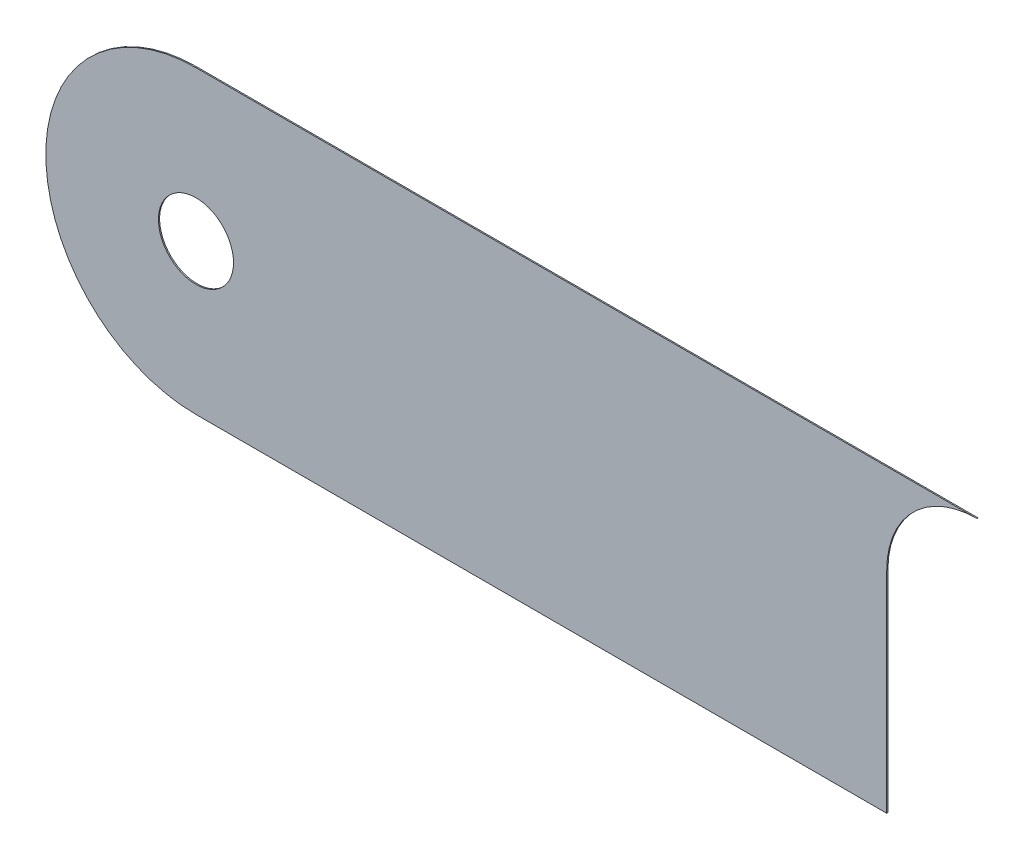
SolidWorks part; units mm, degrees
material "普通碳钢"
ref_plane "Front Plane" through (0, 0, 0) normal (0, 0, 1) x (1, 0, 0)
ref_plane "Top Plane" through (0, 0, 0) normal (0, 1, 0) x (1, 0, 0)
ref_plane "Right Plane" through (0, 0, 0) normal (1, 0, 0) x (0, 0, -1)
sketch "Sketch1" plane through (0, 0, 0) normal (0, 0, 1) x (1, 0, 0)
  line L0 (0, 254) -> (1320.8, 254)
  line L1 (0, -254) -> (1168.4, -254)
  line L2 (1168.4, -254) -> (1168.4, 101.6)
  circle A0 centre (0, 0) radius 63.5
  arc A1 (0, 254) -> (0, -254) centre (0, 0) ccw
  arc A2 (1320.8, 254) -> (1168.4, 101.6) centre (1320.8, 101.6) ccw
  dimension "D1" = 127
  dimension "D2" = 508
  dimension "D3" = 304.8
  dimension "D4" = 152.4
  dimension "D5" = 1320.8
extrude "Boss-Extrude1" add sketch "Sketch1" along normal mid plane 2
